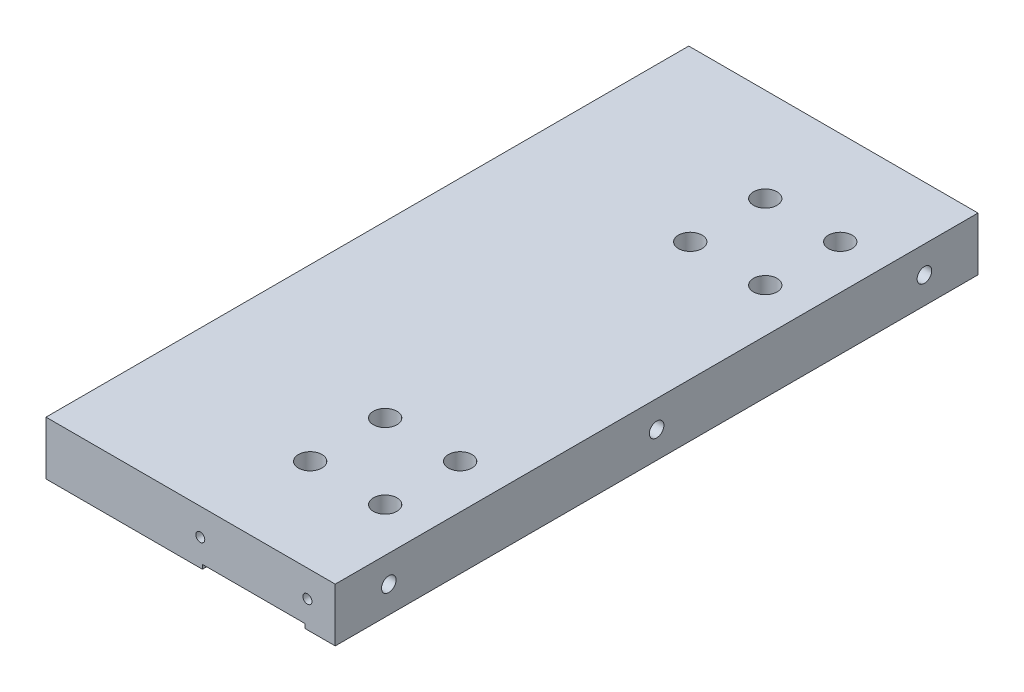
from build123d import *

# Parameters (mm, degrees)
SKETCH_1_W                   = 135
SKETCH_1_H                   = 300
EXTRUDE_1_DEPTH              = 25
SKETCH_2_W                   = 48
SKETCH_2_H                   = 2
CUT_EXTRUDE_1_DEPTH          = 309.514586365
HOLE_WIZARD_M8_1_AT_2_COUNT  = 2
HOLE_WIZARD_M8_1_AT_2_PITCH  = 250
HOLE_WIZARD_M8_1_AT_3_COUNT  = 2
HOLE_WIZARD_M8_1_AT_3_PITCH  = 125
HOLE_WIZARD_M6_1_D           = 6.6
HOLE_WIZARD_M6_1_CBORE_D     = 11
HOLE_WIZARD_M6_1_CBORE_DEPTH = 16.8
HOLE_WIZARD_M5_1_D           = 4.2
HOLE_WIZARD_M5_1_DEPTH       = 12.4
HOLE_WIZARD_M5_1_TIP         = 1.2618073


with BuildPart() as part:
    # 草图1 → 凸台-拉伸1 (new body)
    with BuildSketch(Plane(origin=(0, 0, 0), x_dir=(1, 0, 0), z_dir=(0, 1, 0))):
        Rectangle(SKETCH_1_W, SKETCH_1_H)
    extrude(amount=EXTRUDE_1_DEPTH)

    # 草图2 → 切除-拉伸1 (cut, through all)
    with BuildSketch(Plane.XY.offset(150)):
        with Locations((29.5, 1)):
            Rectangle(SKETCH_2_W, SKETCH_2_H)
    extrude(amount=-CUT_EXTRUDE_1_DEPTH, mode=Mode.SUBTRACT)

    # 草图6 → M8 螺纹孔1 (revolve, cut)
    with BuildSketch(Plane(origin=(-67.5, 12.5, -125), x_dir=(0, 0, 1), z_dir=(0, 1, 0))):
        Polygon((0, 0), (0, 21.792926105), (3.4, 19.75), (3.4, 0), align=None)
    hole_wizard_m8_1 = revolve(axis=Axis((-73.85, 12.5, -125), (1, 0, 0)), mode=Mode.SUBTRACT)

    # M8 螺纹孔1 at 2: M8 螺纹孔1 ×2
    with Locations(*[(0, 0, i * HOLE_WIZARD_M8_1_AT_2_PITCH) for i in range(1, HOLE_WIZARD_M8_1_AT_2_COUNT)]):
        add(hole_wizard_m8_1, mode=Mode.SUBTRACT)

    # M8 螺纹孔1 at 3: M8 螺纹孔1 ×2
    with Locations(*[(0, 0, i * HOLE_WIZARD_M8_1_AT_3_PITCH) for i in range(1, HOLE_WIZARD_M8_1_AT_3_COUNT)]):
        add(hole_wizard_m8_1, mode=Mode.SUBTRACT)

    # 镜向1: M8 螺纹孔1 across plane
    add(hole_wizard_m8_1.mirror(Plane(origin=(0, 0, 0), x_dir=(0, 0, 1), z_dir=(1, 0, 0))), mode=Mode.SUBTRACT)

    # 镜向1 copy 1 sketch → 镜向1 copy 1 (revolve, cut)
    with BuildSketch(Plane(origin=(67.5, 12.5, 125), x_dir=(0, 0, 1), z_dir=(0, 1, 0))):
        Polygon((0, 0), (0, -21.792926105), (3.4, -19.75), (3.4, 0), align=None)
    revolve(axis=Axis((73.85, 12.5, 125), (1, 0, 0)), mode=Mode.SUBTRACT)

    # 镜向1 copy 2 sketch → 镜向1 copy 2 (revolve, cut)
    with BuildSketch(Plane(origin=(67.5, 12.5, 0), x_dir=(0, 0, 1), z_dir=(0, 1, 0))):
        Polygon((0, 0), (0, -21.792926105), (3.4, -19.75), (3.4, 0), align=None)
    revolve(axis=Axis((73.85, 12.5, 0), (1, 0, 0)), mode=Mode.SUBTRACT)

    # M6 六角圆柱头螺钉的柱形沉头孔1 (through all)
    with Locations(Plane(origin=(0, 25, 0), x_dir=(1, 0, 0), z_dir=(0, 1, 0))):
        with Locations((12, -71.2), (47, -71.2), (47, -106.2), (12, -106.2), (12, 71.2), (12, 106.2), (47, 106.2), (47, 71.2)):
            CounterBoreHole(HOLE_WIZARD_M6_1_D / 2, HOLE_WIZARD_M6_1_CBORE_D / 2, HOLE_WIZARD_M6_1_CBORE_DEPTH)

    # M5 螺纹孔1
    with Locations(Plane.XY.offset(150)):
        with Locations((4.5, 12.5), (54.5, 12.5)):
            Hole(HOLE_WIZARD_M5_1_D / 2, depth=HOLE_WIZARD_M5_1_DEPTH)
            with Locations((0, 0, -(HOLE_WIZARD_M5_1_DEPTH + HOLE_WIZARD_M5_1_TIP / 2))):  # 118° drill point
                Cone(0, HOLE_WIZARD_M5_1_D / 2, HOLE_WIZARD_M5_1_TIP, mode=Mode.SUBTRACT)


solid = part.part
